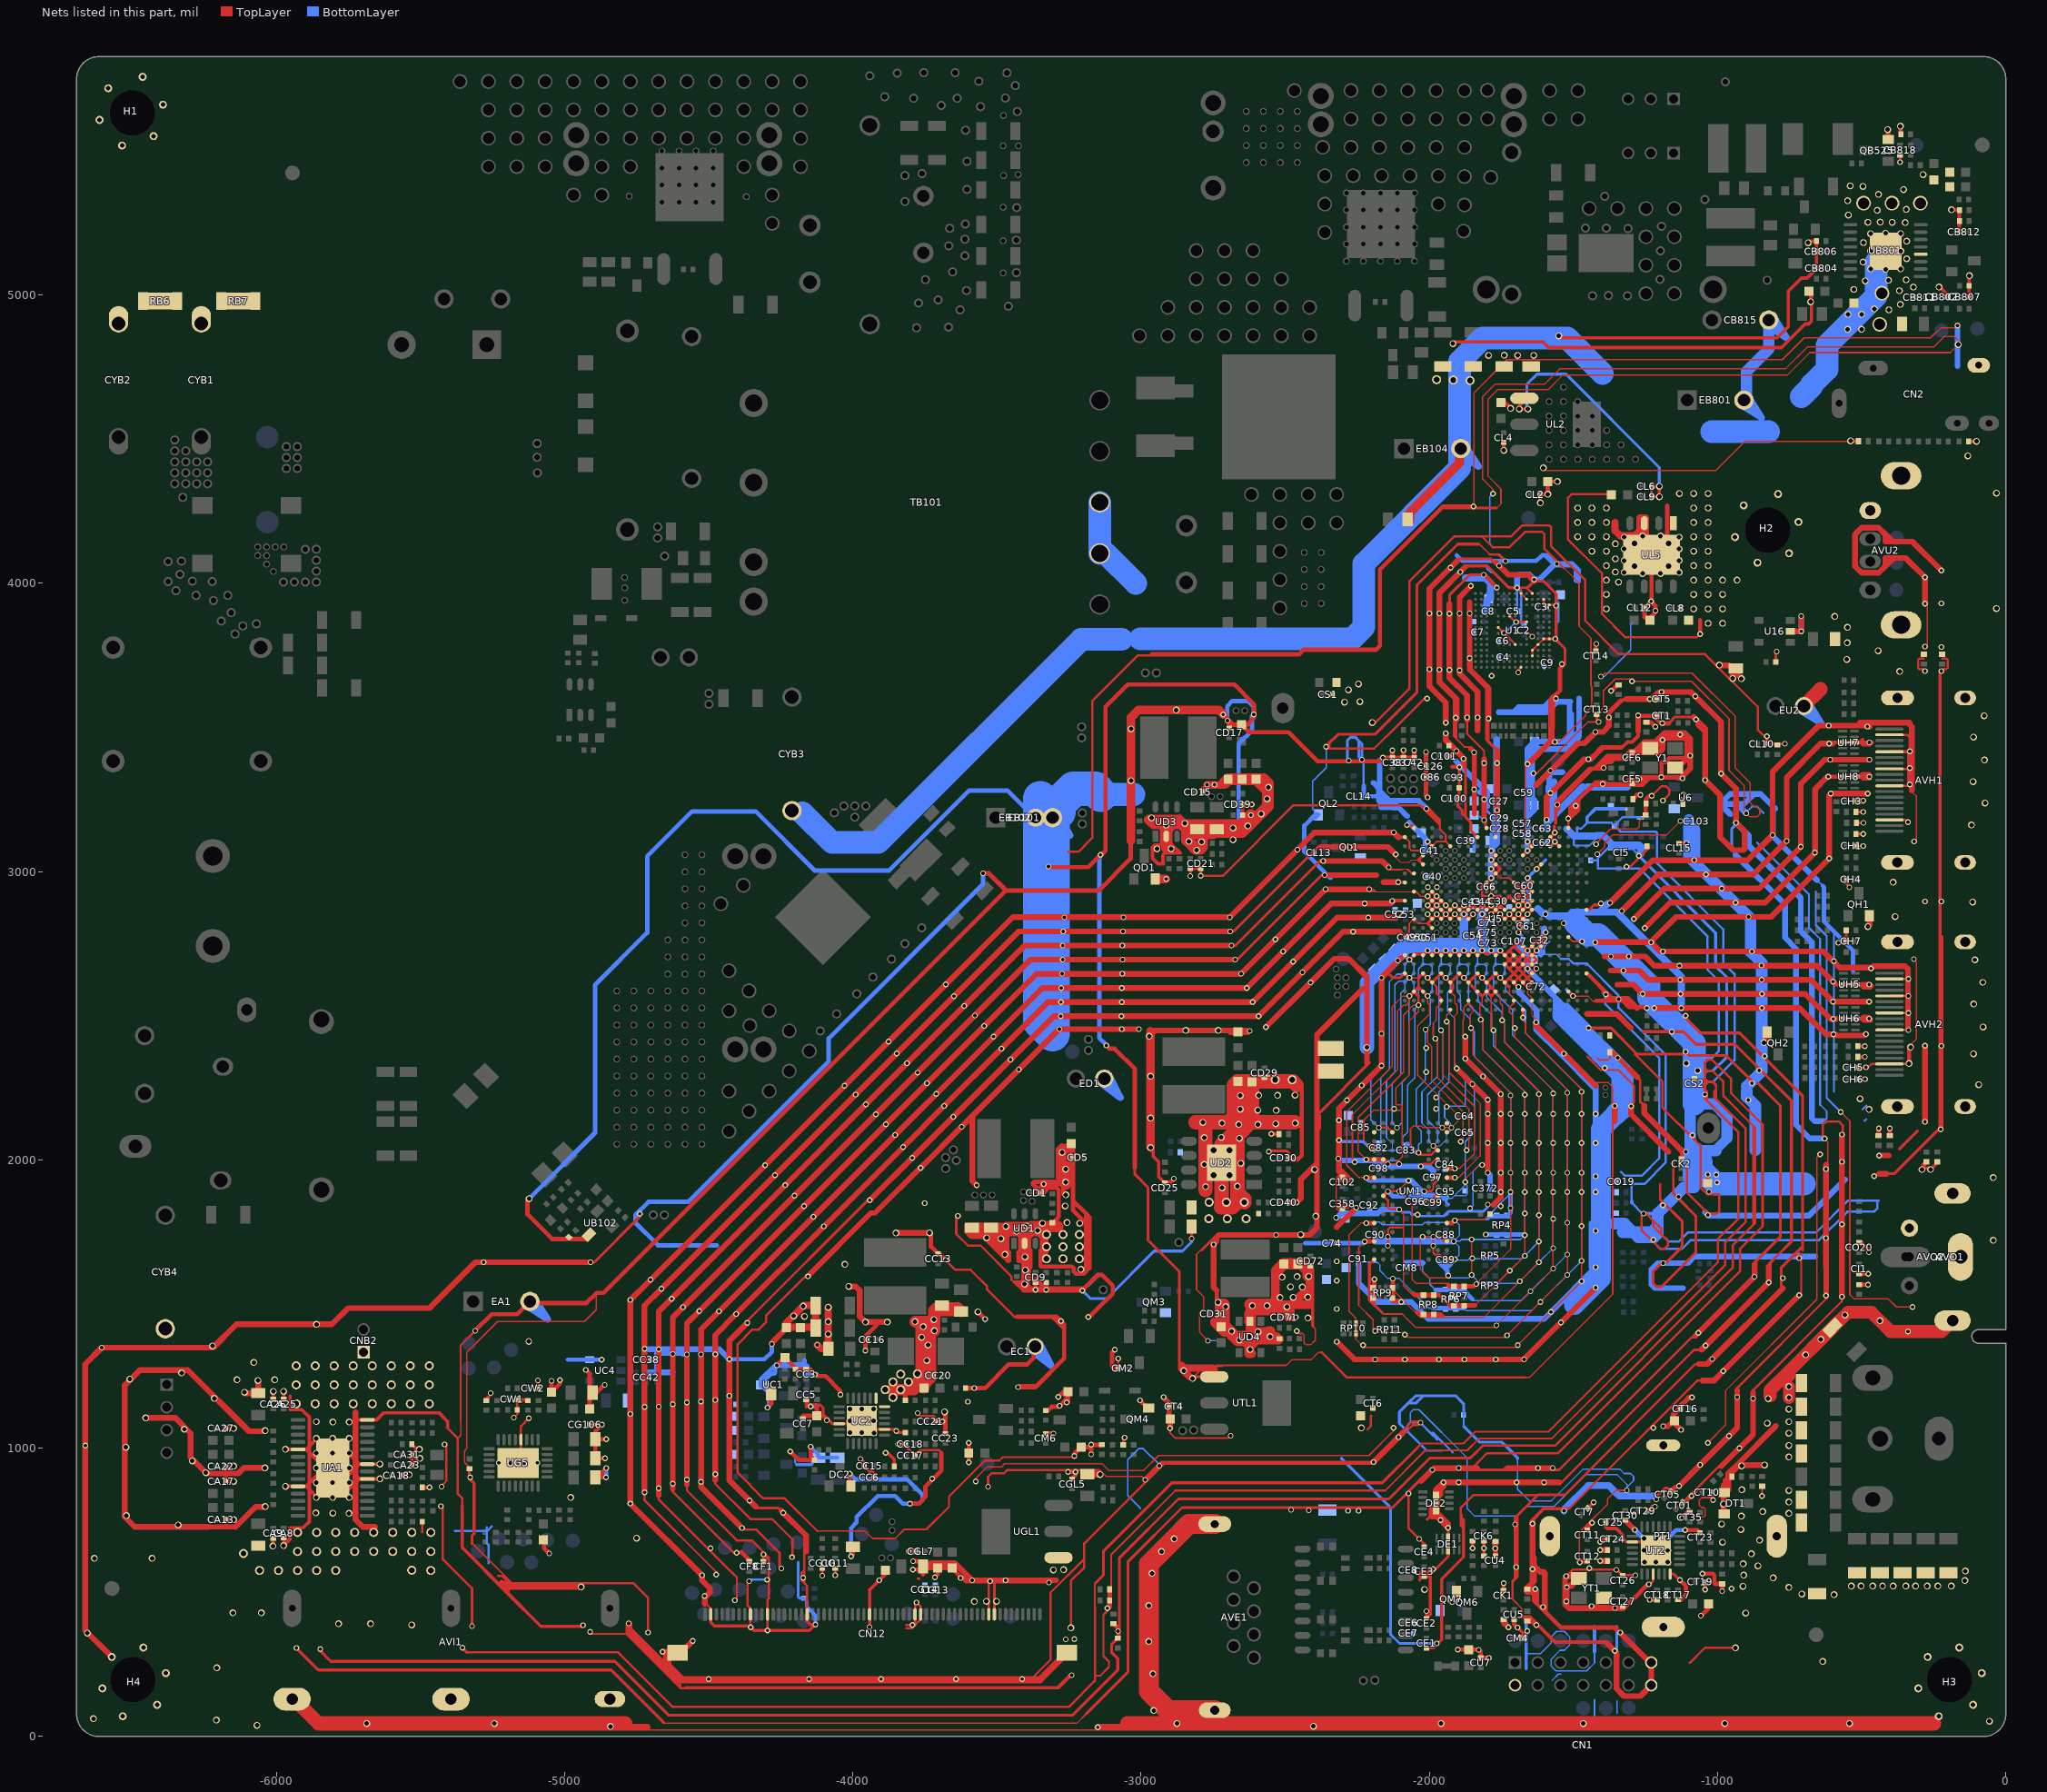
[diagram p0: the nets of this part, all layers, seen from the top]
# Altium PCB MISC84395.PcbDoc (part 17 of 26)
Units mil, origin at the board's own origin, x right, y up, seen from the top; angles counter-clockwise.
Board outline 6692.91 x 5826.77 mil, 2 copper layers (TopLayer, BottomLayer), stack 61.855 mil thick; 951 components, 565 nets, 4374 pads, 1804 vias.
Unrouted connection lines stored in the file: 1.

## Via types
v1: diameter 19.68, hole 11.81, TopLayer to BottomLayer, tented both sides, 1262 vias
v2: diameter 23.62, hole 15.75, TopLayer to BottomLayer, tented both sides, 524 vias
v3: diameter 31.5, hole 19.68, TopLayer to BottomLayer, tented both sides, 11 vias
v4: diameter 24, hole 16, TopLayer to BottomLayer, tented both sides, 6 vias
v5: diameter 19, hole 11.81, TopLayer to BottomLayer, tented both sides, 1 vias

## Nets (pads, with @x,y where several pads share a name; then routed paths per layer and width w, separated by ;. In a path a pad name is that pad's centre, name@x,y a point inside that pad or via, vN(x,y) a via of type N, cw(c..) or ccw(c..) an arc to the next point about the centre after c; other vN are vias at no path point) (continued)
GND: (continued)
  TopLayer w15.75: v2(-5123,1865) -5128,1860 -5128,1811 -5043,1726 -4991,1726 RB134.1@-4984.83,1732.17 -4978.66,1726 -4924.67,1726 UB102.A@-4913.01,1737.66 ; v1(-3548,2994) -3528,2994 -3468,2934 -3437,2934 ; v1(-2224.69,1716.49) -2223.22,1717.97 UM1.P1@-2191.23,1717.97 ; v1(-2218.79,1780.96) UM1.M1@-2191.23,1780.97 ; RP9.8@-2191.23,1512.76 -2191.23,1585.59 v1(-2190.74,1586.08) ; RP9.2@-2126.27,1520.63 RP9.1@-2126.27,1548.68 ; RP9.1@-2126.27,1556.06 RP9.1@-2126.27,1548.68 ; v1(-2097.23,1507.34) -2098.71,1507.34 -2100.68,1509.31 -2126.27,1509.31 RP9.1@-2126.27,1548.68 ; -2055.21,1536.22 -2049.95,1530.97 RP8.1@-2020.46,1530.97 ; -2042.99,1472.32 -2034.7,1464.04 RP8.7@-2020.46,1464.04 ; RP8.7@-2020.46,1465.02 -2020.46,1463.25 RP8.8@-1977.15,1463.25 ; RP8.1@-2020.46,1529.98 RP8.2@-1977.15,1529.98 ; RP8.8@-1985.03,1464.04 -1962.42,1464.04 -1961.63,1463.25 ; RP8.8@-1977.15,1465.02 RP8.8@-1977.15,1463.25 ; -1957.09,1458.7 -1961.63,1463.25 ; UM1.T9@-1939.26,1654.98 v1(-1911.7,1654.98) ; UM1.M9@-1939.26,1780.97 -1920.56,1780.96 v1(-1911.7,1789.82) ; UM1.G9@-1939.26,1938.45 v1(-1911.7,1938.44) ; UM1.F9@-1939.26,1969.94 v1(-1911.7,1969.94) ; -1934.72,1565.83 -1930.37,1561.48 -1924.99,1561.48 -1846.24,1561.48 ; -1924.99,1495.04 -1841.33,1495.04 ; RP8.8@-1977.15,1463.25 -1961.63,1463.25
  TopLayer w18: -6250,726.21 -6249,727.21 -6176.94,727.21 -6140.82,727.21 ; v1(-4155.69,1595.87) -4155.69,1597.06 -3936.92,1815.83 -3922.77,1815.83 -3753.84,1984.76 ; v1(-2922,1177) -2922,1175.5 -2903,1156.5 CT4.2@-2903,1145 CT3.1@-2903,1102 ; v1(-2899.5,1069.5) -2898.81,1070.19 CT3.1@-2898.81,1102 ; -1855.7,3425.34 -1844.82,3414.46 -1843.97,3413.61 -1843.97,3412.41 v1@-1843.97,3285.84 ; v1(-1844.81,3285) v1@-1843.97,3285.84 ; -1843.97,3199.89 v1@-1843.97,3285.84 ; CT30.1@-1321,750.27 v1(-1287.73,717) ; v1(-1189,1076) -1172.81,1076 CT15.1@-1152.81,1096 ; Y1.2@-1148.03,3360.74 -1137.26,3360.74 -1106.47,3391.53 -1106.47,3455.12 -1114.67,3463.32 -1117.02,3463.32 -1118.02,3464.32 ; CT16.1@-1132.73,1141.07 CT16.1@-1132.73,1138 ; v1(-1127,1064) -1152.81,1089.81 CT15.1@-1152.81,1096 ; v1@-1097.8,1176 v1(-1089,1176) -1099.76,1176 -1132.73,1143.04 CT16.1@-1132.73,1138 ; CT15.1@-1152.81,1096 -1152.81,1117.92 CT16.1@-1132.73,1138
  TopLayer w19: -624,1630 -624,1529.5 v1@-623.5,1529
  TopLayer w19.68: -1629.71,2464.52 v1(-1533.75,2368.56) -1422.79,2257.6 ; -1629.71,2464.53 v1(-1629.71,2476.83) ; -1466.01,2300.83 -1454.24,2289.06
  TopLayer w19.69: v1(-2321.15,1369.55) -2259.64,1308.03 v1(-1671.54,1308.03) v1(-1423.02,1556.56) ; -2321.15,1766.69 v1@-2258.65,1829.19 ; -2316.31,1934.42 -2314.49,1932.6 -2276.79,1932.6 -2303.44,1959.25 -2313.77,1959.25 ; C102.2@-2301.47,1946.95 -2313.77,1959.25 ; v1(-2166.13,2631.85) v1(-2166.13,2326.73) -2313.77,2179.09 v1(-2313.77,2137.52) v1(-2313.77,2068.36) -2313.77,1959.25 ; v1@-2166.13,2632.83 -2100.68,2698.28 ; v1(-1905.3,2316.89) v1(-1851.17,2262.75) v1(-1797.04,2208.62) v1(-1797.03,1955.18) ; v1(-1875.78,2427.62) v1(-1875.78,2351.34) v1(-1814.26,2289.82) v1(-1752.75,2228.3) -1752.75,1869.05 -1777.84,1843.95 ; -1629.71,2464.52 v1(-1629.71,2476.83)
  TopLayer w20: H4.2@-6570.6,276.03 -6662.41,367.84 v1(-6662.41,1009) -6662.41,1291.59 v1(-6605.13,1348.87) -6307,1348.87 ; -6481.74,1262.39 -6473,1271.13 ; v2(-6453.08,1105.08) -6350.22,1105.08 -6297,1051.86 -6297,968.06 v2(-6243.94,915) ; -6261.87,1348.87 -6307,1348.87 ; -6236,727.21 -6249,727.21 -6491.21,727.21 -6526,762 -6526,1218.13 -6473,1271.13 ; v2@-6233.94,912.21 -6175.29,912.21 -6132.02,912.21 -6112.23,932 v2(-6039.23,932) ; -6140.82,727.21 -6072.04,796 v2@-6036.44,796 ; v2@-6109.91,1191.03 CA2.1@-6061.94,1191.03 v2@-6061.94,1232 ; v2(-6038.25,797.81) v2@-6036.44,796 ; v2(-6038.25,1060.59) -6040.06,1058.78 -6094.73,1058.78 -6307.08,1271.13 -6473,1271.13 ; v2@-6035.44,796 v2@-6036.44,796 ; -5724.67,1124.28 -5724.67,957.61 -5724.67,931.86 -5724.67,906.43 -5724.67,880.68 -5724.67,752.5 -5699.17,727 -5656.94,727 ; -5218.08,533.5 -5203.58,519 v2(-4942.5,519) ; v1(-4910,1645) v1(-5281,1645) -5309,1645 -5468,1486 -5750.94,1486 -5806.94,1430 v2(-5859.94,1430) -6138.09,1430 -6219.22,1348.87 -6307,1348.87 ; v1(-4722.5,847) v1(-4722.5,1143) v1(-4722.5,1345) -4722.5,1494.11 v1(-4663.97,1552.64) v1(-4269.88,1946.73) v1(-3990.19,2226.42) v1(-3847.61,2369.01) v1(-3649.14,2567.48) -3424.11,2792.5 v1(-3270,2792.5) v1(-3063,2792.5) v1(-2691,2792.5) ; -4673.5,838 v1(-4673.5,861) v1(-4673.5,1144) v1(-4673.5,1343) -4673.5,1473.82 v1(-4234.7,1912.62) v1(-3954.57,2192.75) v1(-3811.98,2335.33) v1(-3613.51,2533.8) -3403.82,2743.5 v1(-3272,2743.5) v1(-3065,2743.5) v1(-2686,2743.5) ; v1(-4660,294) -4611.16,294 CN12.61@-4607.29,290.13 -4596.87,290.13 v1(-4555,332) ; -4624.5,859 v1(-4624.5,877) v1(-4624.5,1153) v1(-4624.5,1327) -4624.5,1453.52 -3383.52,2694.5 v1(-3272,2694.5) v1(-3064,2694.5) v1(-2673.69,2694.5) ; -4575.5,875 v1(-4575.5,891) v1(-4575.5,1159) v1(-4575.5,1325) -4575.5,1433.22 v1(-4532.67,1476.05) v1(-4168.94,1839.78) v1(-3885.27,2123.45) v1(-3742.69,2266.04) v1(-3544.22,2464.51) -3363.22,2645.5 v1(-3274,2645.5) v1(-3065,2645.5) v1(-2653.39,2645.5) v1(-2534.04,2764.85) v1(-2360.29,2938.6) -2215.26,2938.6 v1(-2208.78,2938.6) ; -4513.77,460.64 -4513.84,460.71 -4513.84,481.29 -4495.5,499.63 -4495.5,514.37 -4522.84,541.71 v1(-4522.84,559.29) v1(-4771.5,807.95) v1(-4771.5,1119) v1(-4771.5,1514.41) v1(-4701.4,1584.51) v1(-4028.5,2257.41) v1(-3875.91,2410) v1(-3677.44,2608.47) -3444.41,2841.5 v1(-3266,2841.5) v1(-3061,2841.5) v1(-2692.15,2841.5) v1(-2457.99,3075.66) -2399.04,3134.6 -2122.71,3134.6 -2106.85,3118.74 ; -4477.5,890 v1(-4477.5,910) v1(-4477.5,1168) v1(-4477.5,1326) -4477.5,1392.63 v1(-4404.36,1465.77) v1(-4100.88,1769.25) v1(-3825.25,2044.88) v1(-3682.66,2187.47) v1(-3484.19,2385.94) -3322.63,2547.5 v1(-3278,2547.5) v1(-3067,2547.5) v1(-2612.8,2547.5) v1(-2472.58,2687.72) -2319.69,2840.6 v1(-2212,2840.6) -2114.09,2840.6 ; v1(-4384.5,723.13) -4526.5,865.13 v1(-4526.5,883) v1(-4526.5,1162) v1(-4526.5,1325) -4526.5,1412.93 v1(-4136.68,1802.75) -3342.93,2596.5 v1(-3277,2596.5) v1(-3067,2596.5) v1(-2633.09,2596.5) -2339.99,2889.6 v1(-2224.19,2889.6) v1@-2134.38,2889.6 ; v1(-4365.93,1434.91) -4428.5,1372.33 v1(-4428.5,1182) -4428.5,888.75 v1(-4358.14,818.39) -4336.88,797.13 ; v1(-4280.67,1361.67) -4280.67,1366.23 CC9.2@-4229.54,1417.35 ; v1@-4247.09,781.91 v1(-4241.47,776.28) -4162.16,696.97 -4162.16,641.49 ; CC9.2@-4231.19,1418.81 CC9.2@-4231,1418.81 CC10.2@-4181,1418.81 ; v2(-4014,1561) -3990,1561 -3976.27,1547.27 -3976.27,1457.7 v2(-3956.28,1437.72) -3918,1437.72 v2(-3880.29,1437.72) ; v1(-3941,1859.83) v1(-3794.02,2006.82) v1(-3651.43,2149.4) v1(-3452.96,2347.87) -3302.33,2498.5 v1(-3279,2498.5) v1(-3068,2498.5) v1(-2592.5,2498.5) -2299.4,2791.6 v1(-2264.79,2791.6) -2103.18,2791.6 ; v2(-3850,1746.1) -3851,1747.1 -3734.1,1747.1 v2(-3734,1747) v2@-3732.73,1747 ; v1(-3765.13,1972.07) v1(-3622.54,2114.65) v1(-3424.07,2313.12) v1(-3283.69,2453.5) v1(-3067,2453.5) v1(-3008,2453.5) ; CC19.2@-3755.97,590 -3740.98,590 -3728.98,602 -3646.21,602 v1(-3586.21,542) v1(-3470,542) -3295,542 ; CD4.2@-3604.46,1772.88 -3604.46,1751.46 -3587.76,1734.75 -3543.48,1734.75 -3535.62,1726.88 v2@-3480.74,1672 ; -3585,2146.43 -3585,1926.79 v1(-3570.61,1912.39) ; v2(-3472,1672) v2@-3480.74,1672 ; -3416.56,1710.82 -3416.56,1736.72 -3425.35,1745.5 -3428.88,1745.5 -3457.46,1745.5 -3466.24,1736.72 -3466.24,1684.92 -3460.4,1679.08 -3460.4,1651.67 v2@-3480.74,1672 ; v1(-2985.45,890) v1(-2936.63,938.81) ; v2(-2972,2429) -2967,2434 -2952,2449 v2(-2845,2449) v2(-2732,2449) -2635.88,2449 ; -2738.65,1547.77 -2748.65,1557.77 v1(-2748.65,1706.72) -2738.65,1716.72 -2738.65,1730.87 -2729.86,1739.65 v1(-2532,1739.65) -2415.35,1739.65 -2390.07,1764.93 ; -2690.31,2443.81 CD2.1@-2664,2443.81 v1@-2630.69,2443.81 ; v1(-2567.09,2460.27) v1(-2411.92,2615.45) -2329.36,2698 -2280,2698 -2216.77,2634.77 v2(-2216.77,2390.46) -2216.77,2335.27 ; v1(-2461,1852) -2446,1867 -2446,1931.72 -2390.07,1987.64 ; -2413,1741 -2390.07,1763.93 -2390.07,1764.93 ; -2377,3085.6 v1(-2277,3085.6) -2143.01,3085.6 v1@-2119.4,3061.99 ; v1(-2369,3036.6) -2163.3,3036.6 v1(-2141.04,3014.34) ; v1(-2363,2987.6) -2183.6,2987.6 ; -2315.89,1840.02 -2283.75,1840.02 ; -2231.8,2592.45 -2390.07,2434.18 -2390.07,1987.64 ; v1(-2193.52,952) v1(-2106.92,1038.59) -2092.76,1052.76 ; -2158.86,2963.29 v1(-2107.7,2963.29) ; v1@-2129.06,2894.93 v1@-2126.13,2897.86 ; -2029,886 v1(-1990,925) -1984,931 v1(-1898,931) -1834.37,931 ; v1(-1943.55,3479.64) -1943.55,3455.79 v1(-1906.07,3418.31) v1@-1880.07,3392.31 ; v1@-1943.55,3514.84 v1(-1943.55,3516.74) -1943.55,3586.17 -2000.21,3642.83 v1(-2000.21,3701.74) v1(-2000.21,3895.74) -2000.21,3980.78 v1(-1926.85,4054.14) -1903,4078 ; v1(-1935,724) v1(-1961.45,750.45) -1974.84,763.84 ; -1935,734 -1935,737.99 -1973.49,776.48 -1973.49,827.67 -1961.07,840.09 -1961.49,840.51 -1961.49,857.5 -1951,867.99 v1(-1951,882) ; -1930.21,3928.74 v1(-1930.21,3894.64) v1(-1930.21,3698.94) -1930.21,3671.83 -1869.21,3610.83 v1(-1869.21,3534.74) v1@-1869.21,3526.49 ; v1@-1908.55,3524.15 v1(-1908.55,3533.74) -1908.55,3600.67 ; v1@-1905.21,3527.49 -1905.21,3597.33 -1908.55,3600.67 ; -1876.65,4054.84 -1965.21,3966.29 v1(-1965.21,3895.04) v1(-1965.21,3699.69) -1965.21,3657.33 -1908.55,3600.67 ; -1860.21,3933.74 v1(-1860.21,3895.29) v1(-1860.21,3740.44) -1860.21,3728.74 ; v1(-1856.11,3990.53) -1895.21,3951.43 v1(-1895.21,3895.04) v1(-1895.21,3697.84) -1895.21,3686.32 -1832.71,3623.82 v1(-1832.71,3534.74) -1832.71,3489 ; v1@-1809.97,3179.59 v1(-1809.97,3249.74) v1(-1809.97,3376.34) -1809.97,3389.84 ; v1@-1794.01,3528.46 -1794.01,3634.63 -1795.87,3636.48 -1802.21,3642.82 -1859.74,3700.35 ; v1(-1771.67,652) -1771.01,652.66 DU7.A@-1771.01,677.27 ; -1768.09,4071 -1726.68,4029.58 -1658.22,4029.58 v1@-1641.37,4012.74 ; -1764.97,3201.08 v1(-1764.97,3213.08) v1(-1764.97,3376.34) -1764.97,3420.88 ; DK1.A@-1742.34,406.15 -1742.34,395.28 v1(-1726,379) v1(-1726,379) ; DU5.A@-1660.3,515.98 DU5.A@-1660.83,515.45 ; DU5.A@-1660.14,516.14 -1642.5,533.78 ; DU6.A@-1660,401.27 -1643.52,401.27 v1(-1628.77,386.52) ; DU6.A@-1660,403.27 -1645.52,403.27 ; v1@-1659.97,3370.58 -1577.21,3453.34 -1577.21,3592.74 ; -1642.5,651 -1642.5,625.49 ; -1642.5,652 v1(-1642.5,738) v1@-1642.5,744.88 ; v1(-1636.65,4012.74) v1@-1641.37,4012.74 ; v1@-1636.37,4007.74 v1@-1641.37,4012.74 ; v1(-1633,511) -1633.27,510.73 v1@-1634.73,510.73 ; -1629.97,3299.81 v1(-1579.89,3349.89) -1485.04,3444.74 -1462.75,3444.74 v1(-1423.59,3483.9) -1398.21,3483.9 -1377.21,3504.9 v1(-1377.21,3534.74) ; -1629,467.36 -1629,487.17 ; -1599.5,437.86 -1599.5,567 -1603.5,571 -1615.5,571 -1637.19,592.69 ; v1(-1593.24,3179.9) -1593.24,3258.76 v1(-1579.58,3272.42) -1462.25,3389.74 v1(-1448.65,3389.74) -1439.97,3389.74 -1410.48,3419.23 -1400.81,3428.9 ; -1568.07,3607.16 -1574.65,3600.58 -1574.65,3500.58 -1575.39,3499.83 -1575.39,3460.49 v1(-1564.65,3449.74) ; -1549.04,882 v1(-1697,882) v1(-1898,882) v1(-1951,882) ; v1(-1525.93,555.93) -1488.77,555.93 YT1.2@-1481.31,548.46 ; v1(-1523,518) -1523,518.27 -1518.87,522.4 -1507.37,522.4 YT1.2@-1481.31,548.46 ; YT1.2@-1492.8,548.46 YT1.2@-1489.31,548.46 ; YT1.2@-1475.07,554.7 YT1.2@-1481.31,548.46 ; -1452.89,2506.53 -1349.76,2506.53 -1301.24,2458.01 ; v1(-1424.71,2754.84) v1@-1232.22,2754.84 ; v1@-1406.98,608.98 DT2.A@-1381.9,608.98 ; v1@-1406.98,646.98 DT3.A@-1382.07,646.98 ; -1392.72,2582.75 -1368.82,2558.84 -1312.17,2558.84 -1283.22,2529.9 -1280.22,2526.9 ; -1391.39,2705.84 v1(-1370.39,2705.84) v1(-1308.48,2705.84) -1251.28,2705.84 -1219.33,2673.9 v1(-848,2673.9) -655.53,2673.9 v1@-593.25,2611.62 ; -1383.27,323.39 -1350.14,290.27 -1350.14,165.84 -1324.65,140.35 -1267.97,140.35 CN1.14@-1230.31,178 -1230.32,252.46 v1(-1338.43,360.58) ; v1(-1373.48,2891.61) -1228.19,3036.9 ; -1371.71,2656.84 v1(-1326.65,2656.84) -1271.58,2656.84 -1239.63,2624.9 -1074.31,2624.9 -955.98,2624.9 v1(-847,2624.9) -675.82,2624.9 v1(-599.89,2548.96) v1(-474.21,2548.96) ; -1357.33,2134.17 v1(-1357.33,2187) v1@-1357.33,2188 ; -1353.25,375.39 -1351.25,373.39 ; -1348.52,2607.84 -1291.87,2607.84 v1(-1259.93,2575.9) -1054.02,2575.9 -976.28,2575.9 v1(-846,2575.9) -696.12,2575.9 -608.94,2488.72 v1(-598.83,2488.72) v1@-589.83,2488.72 ; v1(-1332.46,2863.33) -1205.42,2990.37 v1(-1040,2990.37) -876.35,2990.37 v1(-760.43,3106.3) -760.43,3326.13 -642.56,3444 v1(-613,3444) -602,3444 ; -1317,3598 v1(-1236,3598) -1230,3598 -1210.73,3617.27 ; -1305.32,2313.24 -1278.46,2286.38 ; v1@-1300.33,2188.41 v1(-1300.33,2186.41) -1300.33,2177 -1300.33,2157.78 -1170.78,2028.22 ; v1(-1290.67,2835.83) -1185.13,2941.37 v1(-986,2941.37) -856.06,2941.37 v1(-711.43,3086) -711.43,3305.84 -629.49,3387.78 v1(-609.37,3387.78) v1(-473.37,3387.78) ; -1275.91,3485.74 v1(-1275.91,3541.74) ; -1254.99,2188.41 -1254.99,2161.93 -1123.09,2030.03 ; v1(-1253.27,2803.93) -1164.83,2892.37 v1(-938,2892.37) -835.76,2892.37 v1(-662.43,3065.71) -662.43,3285.54 v1@-619.19,3328.78 ; Y1.4@-1234.65,3427.67 Y1.4@-1219.72,3427.67 ; -1225.72,3039.37 v1(-1081,3039.37) -896.65,3039.37 v1(-809.43,3126.6) -809.43,3346.43 -649.57,3506.28 v1(-614.37,3506.28) -484.02,3506.28 v1(-480.53,3502.79) v1@-473.04,3502.79 ; v1(-1220,2526.9) v1(-1125.83,2526.9) -1033.72,2526.9 -996.57,2526.9 v1(-846,2526.9) -716.42,2526.9 -624.6,2435.09 v1(-598,2435.09) -590.64,2435.09 -586.96,2431.4 -490.45,2431.4 v1(-485.38,2436.47) ; v1@-1195.52,3450.61 -1218.46,3427.67 Y1.4@-1219.72,3427.67 ; v1(-1195,3622.84) -1091.97,3622.84 v1(-1077.06,3607.94) -988.15,3519.02 -988.15,3339.88 v1(-988.06,3339.8) -935.99,3287.73 v1(-935.99,3169.07) -906.31,3139.39 -906.31,3079.21 -911.15,3074.37 -946.21,3074.37 -990.99,3119.16 -990.99,3264.95 v1(-1043.06,3317.02) -1043.15,3317.1 -1043.15,3485.58 ; v1@-1191.15,3454.98 v1@-1190.59,3455.54 ; v1(-1191.15,3456.24) -1196.78,3450.61 Y1.4@-1219.72,3427.67 ; -1136.11,3325.02 -1127.5,3325.02 v1@-1121.91,3330.61 ; v1(-1133.7,869.22) v1(-1060.52,942.39) -932.25,1070.66 v1(-932.25,1177) -932.25,1200.72 ; v1(-1121.91,3323.24) v1@-1121.91,3330.61 ; -1118.02,3464.32 -1171.65,3464.32 -1181.8,3464.32 v1@-1190.59,3455.54 ; -1105.47,3451.77 -1095.15,3441.45 ; -1083.72,3536.37 -1083.2,3535.84 v1(-1074.68,3527.33) -1043.15,3495.79 -1043.15,3485.58 ; -1076.29,1390.71 v1(-1067.26,1399.74) v1(-872,1595) -872,1635 ; -1067.83,3510.27 -1043.15,3485.58 ; -1065,1292 -1036.41,1292 v1(-1018.78,1309.63) -779,1549.41 -774,1554.41 ; -1056.7,1341 v1(-823,1574.7) -823,1626.07 ; -1052.5,1235 -1012.8,1235 v1(-980.37,1267.42) v1(-717,1530.8) ; v2(-994,3716) -992.46,3714.46 -959.36,3714.46 CU.2@-949.83,3704.94 ; -986.73,938.06 v1(-924.76,1000.03) -877.25,1047.54 v1(-877.25,1172) -877.25,1192.9 ; DT1.3@-979,771.5 -979,871.55 -962.55,888 ; -972,888 -962.55,897.45 ; DT1.1@-962.55,855.65 -962.55,888 ; v2(-947.88,3669.41) -949.83,3671.36 CU.2@-949.83,3704.94 ; v2(-918,3669) -918,3673.1 CU.2@-949.83,3704.94 ; v2(-839.11,2406.54) -827.5,2418.15 QH2.E@-827.5,2444.03 ; v2(-837,942) v2@-926,942 ; -798.29,1077 -933.29,942 ; U16.2@-747.7,3833 v1(-709.84,3833) v1(-709.84,3886) ; -624,1630 v1(-624,1729) v1(-624,1968) -624,1982.73 ; v1(-569,1525) v1(-569,1777) v1(-569,1993) v1(-569,2087.87) ; CH3.1@-513.91,3244.29 v1@-497.33,3244.29 ; -506.95,3516.5 -340.33,3516.5 ; v2(-479,2809) -473.33,2814.67 QH1.E@-473.33,2847 ; v1(-478.89,3270.28) v1(-607.37,3270.28) -607.56,3270.28 -612.83,3265 v1(-612.83,3045.17) -815.22,2842.78 v1(-893,2842.78) -1144.29,2842.78 v1@-1232.22,2754.84 ; v1@-470.65,2666.52 -576.89,2666.52 -633.26,2722.9 v1(-881,2722.9) -1199.04,2722.9 v1(-1230.98,2754.84) v1@-1232.22,2754.84 ; v1(-468.35,2664.22) -460.25,2672.31 -349.89,2672.31 -339.63,2662.05 -339.63,2627.95 -339.63,2568.9 -339.63,2509.84 v1@-339.63,2450.79 ; -440,1952 -414.73,1952 ; v1(-440,2015) -439.78,2015.22 -406,2015.22 ; -334.33,3516.5 -340.33,3516.5 ; v1(-333.38,3301.79) v1@-333.38,3415.65 ; -325.83,3282 -325.83,3502 -340.33,3516.5 ; v1(-280.83,2132.11) v1(-280.83,2395.65) ; v1(-280.83,3929) v1(-280.83,4020.38) -347.95,4087.5 -389.66,4087.5 ; v1(-223.83,4043.99) -324.34,4144.5 -393.32,4144.5 ; -2390.07,1764.93 -2390.07,1987.64 ; DE2.EPAD@-1977,809.63 -1977,766 -1974.84,763.84 ; DE2.EPAD@-1977,809.63 -1977,856 v1(-1951,882) ; DE2.EPAD@-1977,809.63 -1992.52,794.12 -1992.52,763.84 -1974.84,763.84 ; -1860.21,3728.74 -1859.74,3728.27 -1859.74,3700.35 ; -1860.21,3728.74 -1860.21,3700.82 -1859.74,3700.35 ; DU5.A@-1660.83,515.45 -1642.5,533.78 ; DU5.A@-1660.83,515.45 -1660.83,515 -1660.83,501.13 -1642.96,501.13 -1638.17,496.34 -1629,487.17 ; -1642.5,533.78 v1(-1642.5,581) -1642.5,598 ; -1642.5,598 -1642.5,625.49 ; -1642.5,598 -1637.19,592.69 ; -1642.5,625.49 -1637.19,620.18 -1637.19,592.69 ; -1637.19,592.69 -1637.19,538.14 -1660,515.33 DU5.A@-1660,510.73 v1@-1634.73,510.73 ; v1@-1634.73,510.73 -1629,505 -1629,487.17 ; CF6.2@-1289.05,3413.2 -1289.77,3412.48 CF6.2@-1296.65,3412.48 -1295.92,3413.2 CF6.2@-1289.05,3413.2 ; CF6.2@-1289.05,3413.2 -1253.97,3448.29 -1215.92,3448.29 -1184.24,3479.96 -1114.54,3479.96 -1095.15,3460.56 -1095.15,3448.52 -1095.15,3441.45 ; CF6.2@-1289.05,3413.2 -1287.8,3413.2 -1203,3413.2 -1190.59,3425.61 v1@-1190.59,3455.54 ; v1@-1121.91,3330.61 -1095.15,3357.37 v1(-1095.15,3402.24) -1095.15,3441.45 ; -962.55,888 -962.55,897.45 ; -962.55,897.45 -962.55,912.74 -953.65,921.65 ; -953.65,921.65 -933.29,942 ; -953.65,921.65 -946.35,921.65 v2@-926,942 ; -933.29,942 v2@-926,942 ; -418.36,4058.81 -418.36,4087.5 -389.66,4087.5 ; -418.36,4058.81 -440.98,4036.18 -500.54,4036.18 -523.16,4058.81 -523.16,4169.54 -500.54,4192.17 -440.98,4192.17 -418.36,4169.54 ; -418.36,4058.81 -389.66,4087.5 ; -418.36,4169.54 -418.36,4144.5 -393.32,4144.5 ; -418.36,4169.54 -393.32,4144.5 ; CGL4.1@-3187,910.03 -3185.47,908.5 v2(-3142,908.5) -3150.5,917 -3180.03,917 CGL4.1@-3187,910.03
  TopLayer w24: v2(-5243,45.5) -5230,32.5 -4714,32.5 ; CN12.61@-4641.5,294 -4641.5,246.04 -4592.43,196.97 ; -4606.97,196.97 -4777,367 v1(-4777,392) -4777,358.8 -4615.17,196.97 -3349.88,196.97 CN12.62@-3256.73,290.13 ; v1(-3150.5,32.5) -3032,32.5 -3019,45.5
  TopLayer w25: CC9.2@-4231,1418.81 CC9.2@-4231,1419.81 ; -4155.36,1494.76 v2@-4171.01,1494.76 ; RG8.2@-4141.16,1419.81 CC9.2@-4231,1419.81 ; RG8.2@-4141.16,1423.81 -4129.11,1411.76 RG8.2@-4129.11,1416.76 RG7.2@-4129.11,1492.76 ; RG7.2@-4129.11,1494.76 v2@-4171.01,1494.76 ; v1(-4123.37,1358.63) -4109.74,1345 CC14.1@-4085.06,1345 ; CC14.1@-4085.06,1340 CC14.1@-4085.06,1345 ; v2(-4085.06,1488.94) v2(-4085.06,1439) v2(-4085.06,1396) CC14.1@-4085.06,1345 ; -2859.5,1288 -2849,1277.5 -2752.03,1277.5 -2746.27,1271.73 ; v2(-2852,1269) v2@-2830.55,1247.55 ; v1(-2771,3301) -2745.59,3301 v1(-2745.12,3301.47) ; v1@-2767,3299.5 -2718.88,3299.5 CD19.2@-2711.38,3307 ; -1355.7,4210 -1355.7,4182.75 -1338.45,4165.5 -1286.96,4165.5 -1269.7,4182.75 -1269.7,4226.5 -1249.7,4226.5 -1249.7,4160.5 UL5.EPAD@-1244.2,4155 ; UL5.EPAD@-1229.2,4115.17 UL5.EPAD@-1229.2,4140 ; CC9.2@-4231,1419.81 -4231,1434.78 v2@-4171.01,1494.76
  TopLayer w30: v2(-3404,1569) -3401.15,1571.85 v2@-3401.15,1665.85 ; UD1.2@-3404,1710.82 -3401.15,1707.97 v2@-3401.15,1665.85 ; v2(-3403,1664) v2@-3401.15,1665.85 ; -3341.6,1675 -3336.76,1679.84 -3336.76,1733.02 -3354.24,1750.5 -3378.96,1750.5 -3386.46,1743 -3388.94,1740.52 -3396.44,1733.02 -3396.44,1670.56 v2@-3401.15,1665.85 ; -3034.84,3106.24 v2(-3034.84,3315) v2(-3034.84,3495) -3034.84,3534.98 -3009.83,3560 v2(-2878,3560) -2730,3560 v1(-2715,3545) ; v2(-2967,2043) v2(-2967,2145) v2(-2967,2290) -2967,2434 -2967,2446.5 ; QD1.S@-2950.5,2974.19 v1(-2913.19,2974.19) ; v2@-2730.16,1499 -2730.16,1453.59 -2745,1438.75 -2745,1434.34 -2712.41,1401.75 -2697.97,1401.75 -2686.25,1390.03 -2686.25,1388.21 -2665.94,1367.9 -2639.52,1367.9 -2627.11,1355.49 -2627.11,1327 -2616.62,1327 -2622.21,1332.59 v2(-2622.21,1342) v2@-2622.21,1350.59 ; -2606.98,1481.17 -2616.62,1471.52 -2616.62,1416.39 -2604.91,1404.67 -2564.72,1404.67 -2561.06,1408.32 -2549.32,1408.32 -2549.32,1399.13 -2537.61,1387.42 -2529.29,1387.42 -2521.61,1379.73 -2520,1378.13 -2523,1375.13 -2597.68,1375.13 v2@-2622.21,1350.59 ; -2534.35,1515.58 -2534.35,1610.09 ; -2529.35,1513.51 -2539,1503.87 -2622,1503.87 -2622.21,1503.65 -2622.21,1498.87 -2622.21,1472.65 ; -2415,1614.26 -2415,1560.26 ; v2@-2622.21,1350.59 -2622.21,1388.05 UD4.2@-2622.21,1440.42 -2622.21,1465.93 -2622.21,1472.65 ; -2622.21,1472.65 -2597.3,1497.56 -2545.3,1497.56 -2477.7,1497.56 ; -2477.7,1497.56 -2416.3,1497.56 -2415,1498.86 -2415,1560.26 ; -2477.7,1497.56 -2415,1560.26
  TopLayer w31.5: RB140.2@-2068.81,4217 -2068.81,4244.19 -1895.57,4417.43 EB104.2@-1895.57,4477
  TopLayer w40: -3863.61,1203.39 -3788,1203.39 ; v2(-3784.01,1438.91) -3756,1438.91 ; -3780,1225 -3763.14,1241.86 -3763.14,1252 -3763.14,1431.77 -3756,1438.91 ; CC22.2@-3753.62,1209 -3753.62,1220.23 -3730.86,1242.99 -3730.86,1252 -3730.86,1284.14 ; -3738,1277 -3730.86,1284.14 ; -3730.86,1438.91 -3730.86,1284.14 ; v2(-3716.84,1407.61) v2@-3716.84,1446 ; -3716.84,1460.36 v2@-3716.84,1446 ; CC8.2@-3699.61,1477.6 CC12.2@-3627.6,1477.6 ; CC12.2@-3624,1474 CC12.2@-3627.6,1477.6 ; CD4.2@-3589.86,1762.69 v2@-3470.3,1762.69 ; v2(-3486.62,1726.38) -3494.64,1734.41 -3529,1734.41 -3476.24,1681.65 -3476.24,1740.86 -3461.6,1755.5 ; v2@-3429.5,1755.5 -3461.6,1755.5 ; -3418.64,1752.94 -3406.56,1740.86 UD1.2@-3406.56,1729 ; -3404,1741.4 -3402.4,1743 -3392.46,1752.94 -3382.72,1762.69 ; -3376.91,1768.5 v2@-3340,1768.5 ; -3288.5,1768.5 v2@-3340,1768.5 ; v2@-3262,1916 v2(-3262,1923) v2(-3262,1968) -3262,2037.19 ; -2961.73,3172.94 -2961.73,3178 -2871.6,3178 -2860.29,3166.69 ; UD3.2@-2913,3122.01 pad.VIA5@-2913,3161 -2913,3170.19 pad.VIA5@-2908,3165.19 ; -2910.44,3081.99 -2910.44,3162.75 pad.VIA5@-2908,3165.19 ; CD19.2@-2711.38,3307 CD19.2@-2698,3320.38 CD18.2@-2650,3320.38 -2574.8,3320.38 -2560,3305.57 -2560,3226.43 -2648.74,3137.69 -2746.08,3137.69 -2751,3132.77 -2772.86,3132.77 -2787.5,3118.13 -2787.5,3086 -2795.21,3078.29 -2809.06,3078.29 -2810.46,3078.3 pad.VIA5@-2840.76,3108.6 ; v2(-2681,3151) -2798.35,3151 pad.VIA5@-2840.76,3108.6 ; -2673,1388.26 -2673.85,1388.26 ; v2@-2622.21,1388.05 v2(-2623,1387.26) -2672.85,1387.26 -2673.85,1388.26 ; UD4.2@-2622.21,1440.42 -2621.62,1441.01 -2621.62,1466.52 ; -2622.21,1465.93 -2621.62,1466.52 ; v2@-2622.21,1498.87 v2@-2605,1498.87 ; v1(-2619.13,3195.87) -2653.97,3161.03 pad.VIA5@-2855.5,3161.03 ; -2616.62,1471.52 -2621.62,1466.52 ; -2601,1487.14 -2555.72,1487.14 -2545.3,1497.56 -2539,1503.87 ; CD45.2@-2601,3320.19 -2563.81,3283 v2@-2561,3283 ; -2598.94,1481.17 -2606.98,1481.17 -2552.93,1481.17 -2545,1489.1 -2502.25,1489.1 -2487.61,1474.46 CD71.1@-2487.61,1459.85 ; -2529.35,1615.09 CD74.2@-2505,1639.45 CD73.2@-2456,1639.45 -2443.51,1639.45 -2420,1615.96 v2@-2420,1597 ; v2@-752.76,1173.79 v2(-752.76,1213.79) v2@-752.76,1214.24 ; -3756,1438.91 -3734.38,1438.91 -3719,1454.29 -3719,1476.97 -3709.97,1486 CC8.2@-3693.8,1486 ; v2@-3716.84,1446 -3716.84,1462.95 CC8.2@-3693.8,1486 ; CC8.2@-3693.8,1486 -3636,1486 CC12.2@-3627.6,1477.6 ; v2@-3470.3,1762.69 -3466.99,1766 -3451.1,1766 ; v2@-3470.3,1762.69 -3454.42,1762.69 ; -3461.6,1755.5 -3454.42,1762.69 ; -3454.42,1762.69 -3451.1,1766 ; -3454.42,1762.69 -3382.72,1762.69 ; -3451.1,1766 -3379.4,1766 ; -3382.72,1762.69 -3379.4,1766 ; -3379.4,1766 -3342.5,1766 v2@-3340,1768.5 ; pad.VIA5@-2908,3165.19 -2891.53,3165.19 -2890.03,3166.69 -2861.17,3166.69 pad.VIA5@-2855.5,3161.03 ; pad.VIA5@-2855.5,3161.03 -2840.76,3146.28 pad.VIA5@-2840.76,3108.6 ; CD69.1@-2712.21,1426.62 -2673.85,1388.26 ; CD69.1@-2712.21,1426.62 -2725.16,1439.56 -2725.16,1498.87 -2712.21,1498.87 CD69.1@-2712.21,1426.62
  TopLayer w45: -818,1182 -818,1201.52 -752.76,1266.75 ; -752.76,1252.06 -752.76,1266.75 ; AVO2.4@-185.04,1442.91 -222.95,1405 -400,1405 -467,1472 -547.95,1472 -598.79,1421.16 -598.79,1420.73 -752.76,1266.75